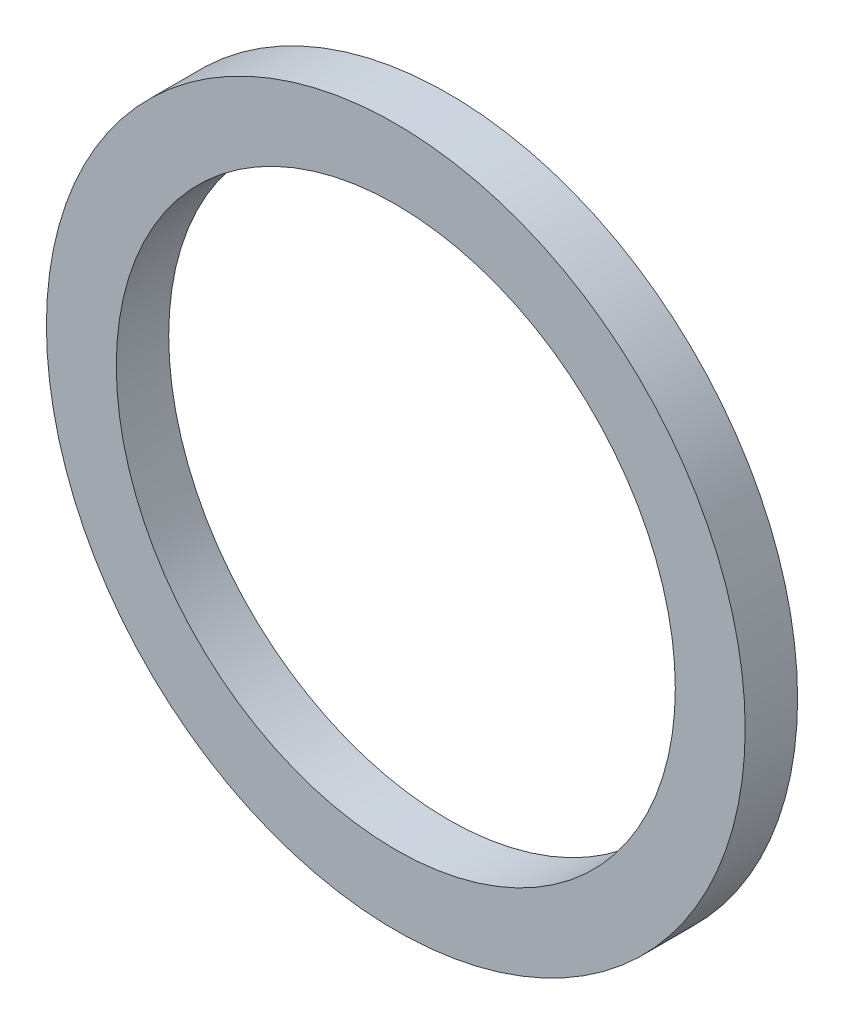
SolidWorks part; units mm, degrees
ref_plane "前视基准面" through (0, 0, 0) normal (0, 0, 1) x (1, 0, 0)
ref_plane "上视基准面" through (0, 0, 0) normal (0, 1, 0) x (1, 0, 0)
ref_plane "右视基准面" through (0, 0, 0) normal (1, 0, 0) x (0, 0, -1)
sketch "草图1" plane through (0, 0, 0) normal (0, 0, 1) x (1, 0, 0)
  circle A0 centre (0, 0) radius 10
  circle A1 centre (0, 0) radius 8
  dimension "D1" = 20
  dimension "D2" = 16
extrude "凸台-拉伸1" add sketch "草图1" along normal blind 1.5
